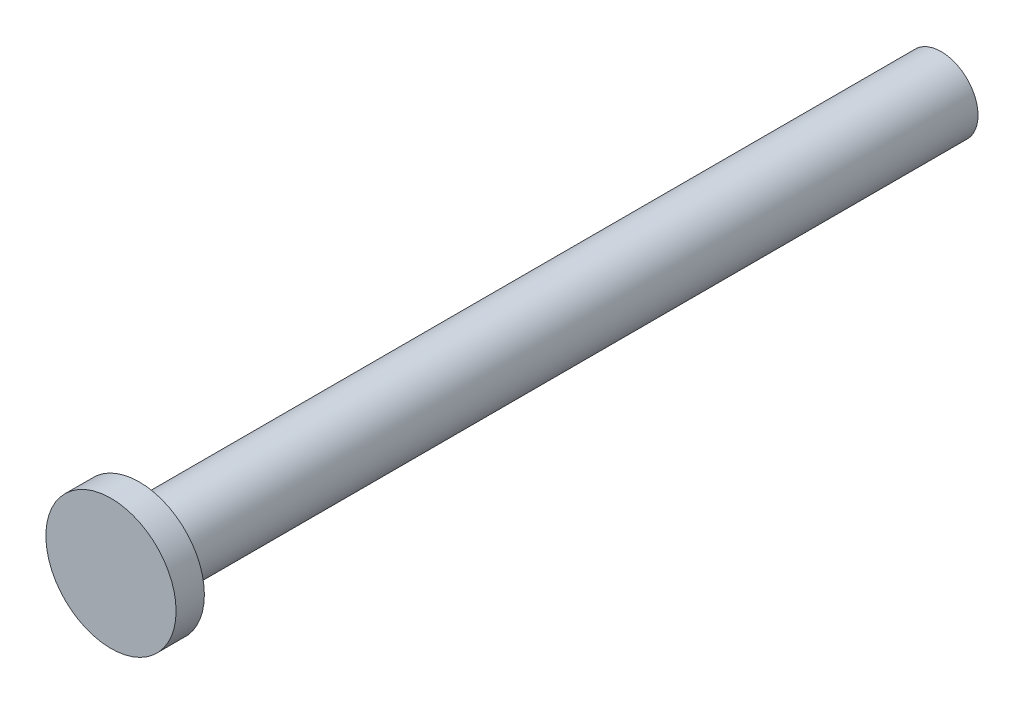
SolidWorks part; units mm, degrees
ref_plane "Front Plane" through (0, 0, 0) normal (0, 0, 1) x (1, 0, 0)
ref_plane "Top Plane" through (0, 0, 0) normal (0, 1, 0) x (1, 0, 0)
ref_plane "Right Plane" through (0, 0, 0) normal (1, 0, 0) x (0, 0, -1)
sketch "Sketch1" plane through (0, 0, 0) normal (0, 0, 1) x (1, 0, 0)
  circle A0 centre (-0.6135, -35) radius 3.9
  dimension "D1" = 7.8
extrude "Boss-Extrude1" add sketch "Sketch1" against normal blind 50 and the other way blind 38
sketch "Sketch2" plane through (0, 0, 38) normal (0, 0, 1) x (1, 0, 0)
  circle A2 centre (-0.6135, -35) radius 6.9
  circle A3 centre (-0.6135, -35) radius 6.9
  dimension "D1" = 3
extrude "Boss-Extrude2" add sketch "Sketch2" against normal up to surface (3 mm away)
